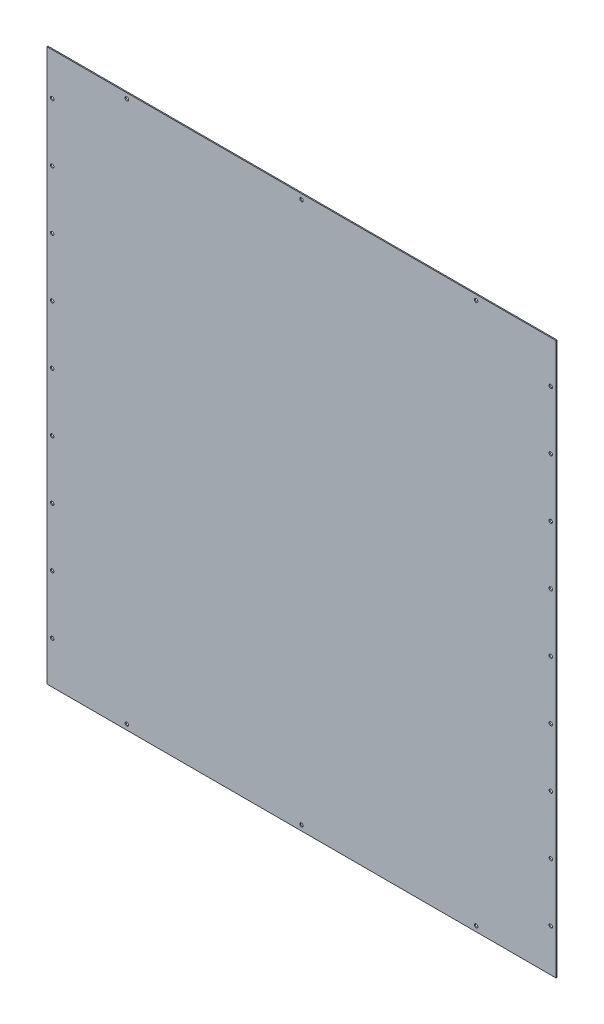
from build123d import *

# Parameters (mm, degrees)
SKETCH_1_W      = 962
SKETCH_1_H      = 1043
SKETCH_1_R      = 3.25
EXTRUDE_1_DEPTH = 2


with BuildPart() as part:
    # 草图1 → 凸台-拉伸1 (new body)
    with BuildSketch(Plane.XY):
        Rectangle(SKETCH_1_W, SKETCH_1_H)
        with Locations((-471, 0)):
            Circle(SKETCH_1_R, mode=Mode.SUBTRACT)
        with Locations((-471, -110.375)):
            Circle(SKETCH_1_R, mode=Mode.SUBTRACT)
        with Locations((-471, -220.75)):
            Circle(SKETCH_1_R, mode=Mode.SUBTRACT)
        with Locations((-471, -331.125)):
            Circle(SKETCH_1_R, mode=Mode.SUBTRACT)
        with Locations((-471, -441.5)):
            Circle(SKETCH_1_R, mode=Mode.SUBTRACT)
        with Locations((0, -511.5)):
            Circle(SKETCH_1_R, mode=Mode.SUBTRACT)
        with Locations(Location((0, 511.5, 0), (0, 0, 180))):
            Circle(SKETCH_1_R, mode=Mode.SUBTRACT)
        with Locations(Location((-471, 441.5, 0), (0, 0, 180))):
            Circle(SKETCH_1_R, mode=Mode.SUBTRACT)
        with Locations(Location((-471, 331.125, 0), (0, 0, 180))):
            Circle(SKETCH_1_R, mode=Mode.SUBTRACT)
        with Locations(Location((-471, 220.75, 0), (0, 0, 180))):
            Circle(SKETCH_1_R, mode=Mode.SUBTRACT)
        with Locations(Location((-471, 110.375, 0), (0, 0, 180))):
            Circle(SKETCH_1_R, mode=Mode.SUBTRACT)
        with Locations((471, 110.375)):
            Circle(SKETCH_1_R, mode=Mode.SUBTRACT)
        with Locations((471, 220.75)):
            Circle(SKETCH_1_R, mode=Mode.SUBTRACT)
        with Locations((471, 331.125)):
            Circle(SKETCH_1_R, mode=Mode.SUBTRACT)
        with Locations((471, 441.5)):
            Circle(SKETCH_1_R, mode=Mode.SUBTRACT)
        with Locations(Location((471, -441.5, 0), (0, 0, 180))):
            Circle(SKETCH_1_R, mode=Mode.SUBTRACT)
        with Locations(Location((471, -331.125, 0), (0, 0, 180))):
            Circle(SKETCH_1_R, mode=Mode.SUBTRACT)
        with Locations(Location((471, -220.75, 0), (0, 0, 180))):
            Circle(SKETCH_1_R, mode=Mode.SUBTRACT)
        with Locations(Location((471, -110.375, 0), (0, 0, 180))):
            Circle(SKETCH_1_R, mode=Mode.SUBTRACT)
        with Locations(Location((471, 0, 0), (0, 0, 180))):
            Circle(SKETCH_1_R, mode=Mode.SUBTRACT)
        with Locations((330, -511.5)):
            Circle(SKETCH_1_R, mode=Mode.SUBTRACT)
        with Locations((-330, -511.5)):
            Circle(SKETCH_1_R, mode=Mode.SUBTRACT)
        with Locations(Location((-330, 511.5, 0), (0, 0, 180))):
            Circle(SKETCH_1_R, mode=Mode.SUBTRACT)
        with Locations(Location((330, 511.5, 0), (0, 0, 180))):
            Circle(SKETCH_1_R, mode=Mode.SUBTRACT)
    extrude(amount=EXTRUDE_1_DEPTH)


solid = part.part
